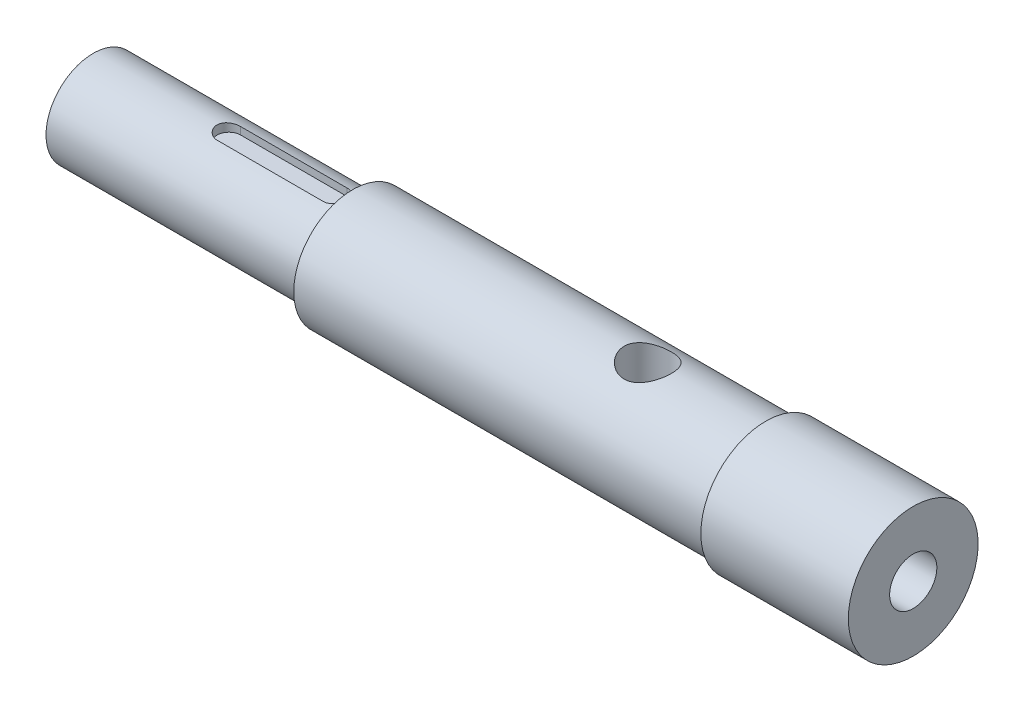
from build123d import *

# Parameters (mm, degrees)
CUT_EXTRUDE1_START      = 8
CUT_EXTRUDE1_DEPTH      = 1.5
CUT_EXTRUDE2_DEPTH      = 140.867794721
CUT_EXTRUDE2_DEPTH_BACK = 140.867794721
SKETCH3_R               = 4


with BuildPart() as part:
    # Sketch1 → Revolve2 (revolve)
    with BuildSketch(Plane.XY, mode=Mode.PRIVATE) as revolve2_sk:
        Polygon((0, 8), (44, 8), (44, 10), (114, 10), (114, 11), (139, 11), (139, 4), (94, 4), (94, 0), (0, 0), align=None)
    revolve(revolve2_sk.sketch.rotate(Axis((0, 0, 0), (1, 0, 0)), 90), axis=Axis((0, 0, 0), (1, 0, 0)))

    # Sketch2 → Cut-Extrude1 (cut)
    with BuildSketch(Plane(origin=(0, 0, 0), x_dir=(1, 0, 0), z_dir=(0, 1, 0)).offset(CUT_EXTRUDE1_START)):
        with BuildLine():
            Line((23, 2), (41, 2))
            ThreePointArc((41, 2), (43, 0), (41, -2))
            Line((41, -2), (23, -2))
            ThreePointArc((23, -2), (21, 0), (23, 2))
        make_face()
    extrude(amount=-CUT_EXTRUDE1_DEPTH, mode=Mode.SUBTRACT)

    # Sketch3 → Cut-Extrude2 (cut, two sides: drawn at the far end of the back side and taken through both)
    with BuildSketch(Plane(origin=(0, 0, 0), x_dir=(1, 0, 0), z_dir=(0, 1, 0)).offset(-CUT_EXTRUDE2_DEPTH_BACK)):
        with Locations(Location((94, 0, 0), (0, 0, 270))):
            Circle(SKETCH3_R)
    extrude(amount=CUT_EXTRUDE2_DEPTH + CUT_EXTRUDE2_DEPTH_BACK, mode=Mode.SUBTRACT)


solid = part.part
